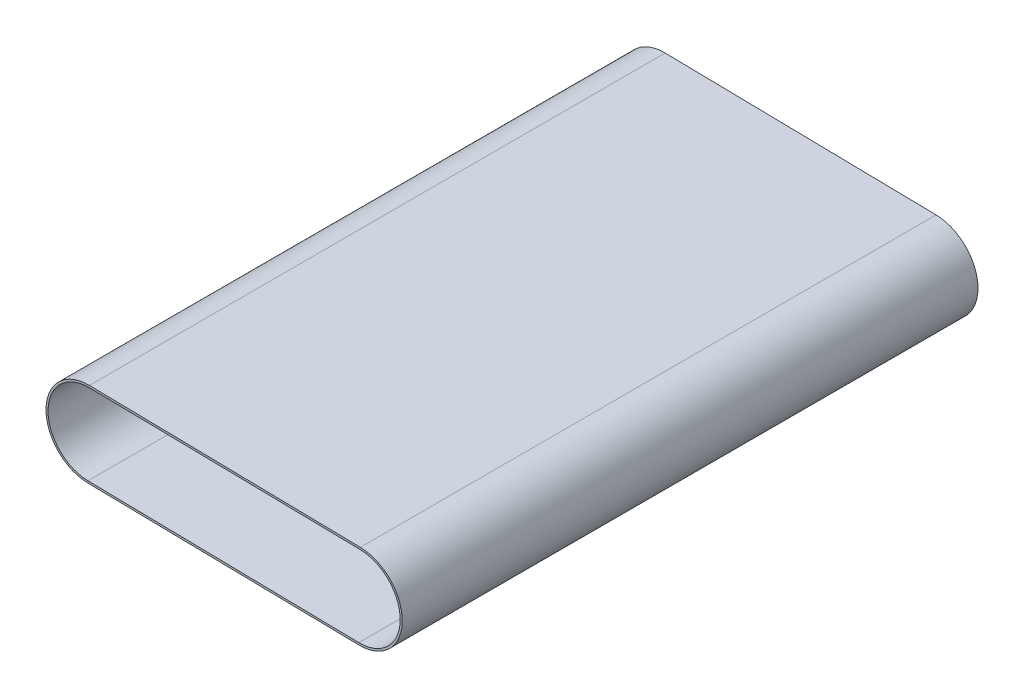
SolidWorks part; units mm, degrees
ref_plane "前视基准面" through (0, 0, 0) normal (0, 0, 1) x (1, 0, 0)
ref_plane "上视基准面" through (0, 0, 0) normal (0, 1, 0) x (1, 0, 0)
ref_plane "右视基准面" through (0, 0, 0) normal (1, 0, 0) x (0, 0, -1)
sketch "草图1" plane through (0, 0, 425) normal (0, 0, -1) x (-1, 0, 0)
  line L0 (-600.9862, 1584.0099) -> (-201.0471, 1590.9909)
  line L1 (-598.8919, 1464.0282) -> (-198.9529, 1471.0091)
  line L2 (-601.0386, 1587.0094) -> (-201.0995, 1593.9904)
  line L3 (-598.8396, 1461.0286) -> (-198.9005, 1468.0096)
  circle A0 centre (-200, 1531) radius 60 construction
  arc A1 (-198.9529, 1471.0091) -> (-201.0471, 1590.9909) centre (-200, 1531) ccw
  circle A3 centre (-599.9391, 1524.019) radius 60 construction
  arc A4 (-600.9862, 1584.0099) -> (-598.8919, 1464.0282) centre (-599.9391, 1524.019) ccw
  arc A5 (-198.9005, 1468.0096) -> (-201.0995, 1593.9904) centre (-200, 1531) ccw
  arc A6 (-601.0386, 1587.0094) -> (-598.8396, 1461.0286) centre (-599.9391, 1524.019) ccw
  dimension "D1" = 3
extrude "凸台-拉伸1" add sketch "草图1" along normal up to surface (850 mm away)
